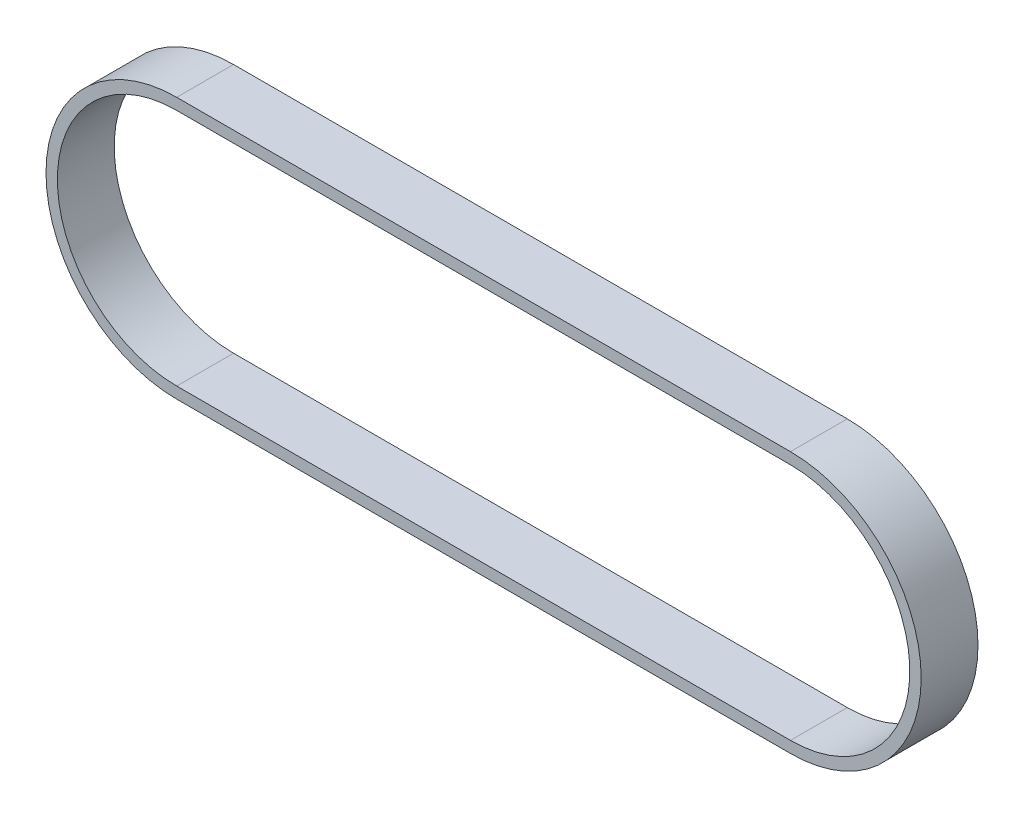
SolidWorks part; units mm, degrees
ref_plane "前视基准面" through (0, 0, 0) normal (0, 0, 1) x (1, 0, 0)
ref_plane "上视基准面" through (0, 0, 0) normal (0, 1, 0) x (1, 0, 0)
ref_plane "右视基准面" through (0, 0, 0) normal (1, 0, 0) x (0, 0, -1)
sketch "草图1" plane through (0, 0, 0) normal (0, 0, 1) x (1, 0, 0)
  line L0 (0, 0) -> (108, 0) construction
  line L1 (0, 21) -> (108, 21)
  line L2 (0, -21) -> (108, -21)
  arc A0 (0, 21) -> (0, -21) centre (0, 0) ccw
  arc A1 (108, -21) -> (108, 21) centre (108, 0) ccw
  point P3 (54, 0)
  dimension "D1" = 42
  dimension "D2" = 108
extrude "拉伸-薄壁1" add sketch "草图1" along normal mid plane 10 thin thin type one direction wall 2
